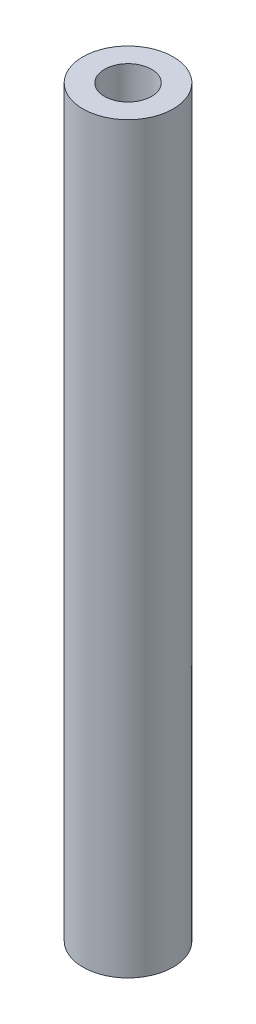
SolidWorks part; units mm, degrees
material "45"
ref_plane "Front Plane" through (0, 0, 0) normal (0, 0, 1) x (1, 0, 0)
ref_plane "Top Plane" through (0, 0, 0) normal (0, 1, 0) x (1, 0, 0)
ref_plane "Right Plane" through (0, 0, 0) normal (1, 0, 0) x (0, 0, -1)
sketch "Sketch1" plane through (0, 0, 0) normal (1, 0, 0) x (0, 0, -1)
  line L0 (0, 0) -> (0, 395) construction
  line L1 (0, 395) -> (24, 395)
  line L2 (24, 395) -> (24, 0)
  line L3 (24, 0) -> (9.25, 0)
  line L4 (9.25, 0) -> (9.25, 5)
  line L5 (9.25, 5) -> (11.5, 5)
  line L6 (11.5, 5) -> (11.5, 8)
  line L7 (11.5, 8) -> (0, 8)
  line L8 (0, 8) -> (0, 395)
  point P3 (10.375, 5)
  dimension "D1" = 24
  dimension "D2" = 11.5
  dimension "D3" = 9.25
  dimension "D4" = 5
  dimension "D5" = 3
  dimension "D6" = 395
revolve "Revolve1" add sketch "Sketch1" angle 360 about L0
sketch "Sketch2" plane through (0, 395, 0) normal (0, 1, 0) x (1, 0, 0)
  point P0 (0, 0)
hole_wizard "Ø25.0 (25) Diameter Hole1" positions "3DSketch1" profile "Sketch3" hole size "Ø25.0" standard "GB"
sketch3d "3DSketch1"
  point P0 (0, 395, 0)
sketch "Sketch3" plane through (0, 395, 0) normal (1, 0, 0) x (0, 0, 1)
  line L0 (0, 0) -> (0, 37.5108)
  line L1 (0, 37.5108) -> (12.5, 30)
  line L2 (12.5, 30) -> (12.5, 0)
  line L5 (12.5, 0) -> (0, 0)
  line L10 (0, 37.5108) -> (-12.5, 30) construction
  line L11 (0, -6.35) -> (0, 107.95) construction
  dimension "孔直径" = 25
  dimension "孔深度" = 30
  dimension "导头角度" = 118
